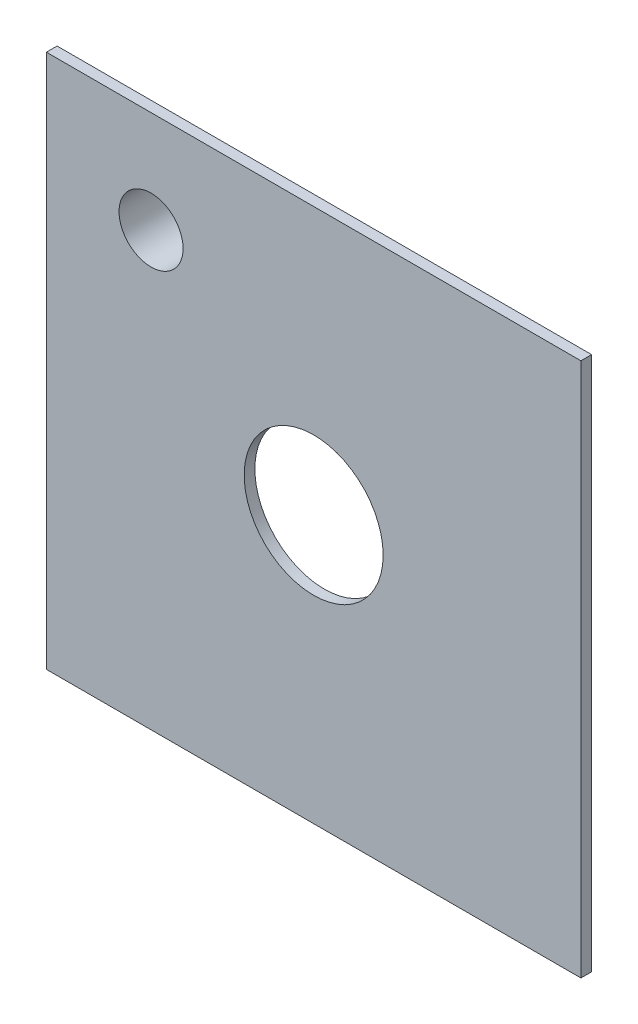
from build123d import *

# Parameters (mm, degrees)
SKETCH1_W           = 500
SKETCH1_H           = 500
SKETCH1_R           = 65
SKETCH1_R_2         = 30
BOSS_EXTRUDE1_DEPTH = 10
SKETCH2_R           = 35
SKETCH2_R_2         = 29.957117648
BOSS_EXTRUDE2_DEPTH = 50


with BuildPart() as part:
    # Sketch1 → Boss-Extrude1 (new body)
    with BuildSketch(Plane.XY):
        with Locations((250, 250)):
            Rectangle(SKETCH1_W, SKETCH1_H)
        with Locations((250, 250)):
            Circle(SKETCH1_R, mode=Mode.SUBTRACT)
        with Locations((97.913524384, 404.851684263)):
            Circle(SKETCH1_R_2, mode=Mode.SUBTRACT)
    extrude(amount=BOSS_EXTRUDE1_DEPTH)

    # Sketch2 → Boss-Extrude2 (add)
    with BuildSketch(Plane.XY.offset(10)):
        with Locations((97.913524384, 404.851684263)):
            Circle(SKETCH2_R)
        with Locations((97.913524384, 404.851684263)):
            Circle(SKETCH2_R_2, mode=Mode.SUBTRACT)
    extrude(amount=-BOSS_EXTRUDE2_DEPTH)


solid = part.part
